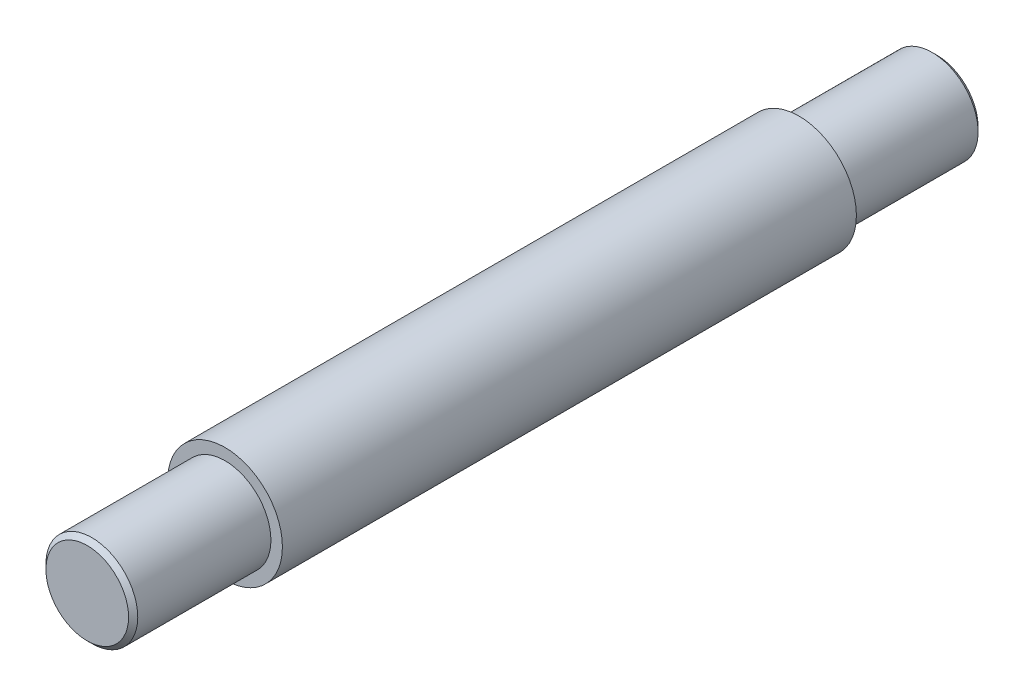
SolidWorks part; units mm, degrees
ref_plane "Front Plane" through (0, 0, 0) normal (0, 0, 1) x (1, 0, 0)
ref_plane "Top Plane" through (0, 0, 0) normal (0, 1, 0) x (1, 0, 0)
ref_plane "Right Plane" through (0, 0, 0) normal (1, 0, 0) x (0, 0, -1)
sketch "Sketch1" plane through (0, 0, 0) normal (0, 0, 1) x (1, 0, 0)
  circle A0 centre (0, 0) radius 12.5
  dimension "D1" = 25
extrude "Boss-Extrude1" add sketch "Sketch1" along normal mid plane 125
sketch "Sketch2" plane through (0, 0, 62.5) normal (0, 0, 1) x (1, 0, 0)
  circle A0 centre (0, 0) radius 10
extrude "Boss-Extrude2" add sketch "Sketch2" along normal blind 30
sketch "Sketch3" plane through (0, 0, -62.5) normal (0, 0, -1) x (-1, 0, 0)
  circle A0 centre (0, 0) radius 10
extrude "Boss-Extrude3" add sketch "Sketch3" along normal blind 30
chamfer "Chamfer1" distance 1 angle 45 2 edges at (10, 0, 92.5) (-10, 0, -92.5)
